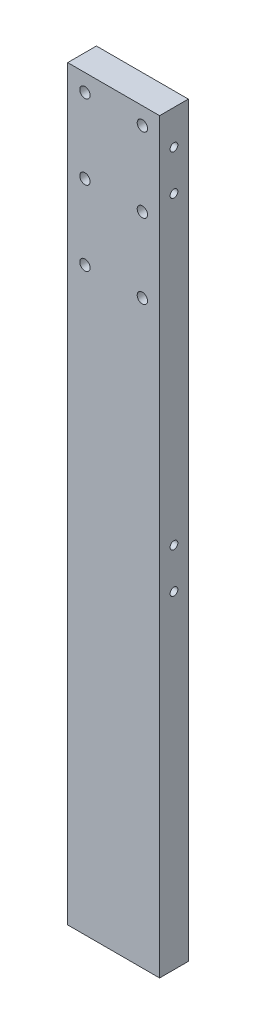
SolidWorks part; units mm, degrees
material "普通碳钢"
ref_plane "Front Plane" through (0, 0, 0) normal (0, 0, 1) x (1, 0, 0)
ref_plane "Top Plane" through (0, 0, 0) normal (0, 1, 0) x (1, 0, 0)
ref_plane "Right Plane" through (0, 0, 0) normal (1, 0, 0) x (0, 0, -1)
sketch "Sketch1" plane through (0, 0, 0) normal (0, 0, 1) x (1, 0, 0)
  line L0 (80, 0) -> (80, 80)
  line L1 (0, 0) -> (80, 0)
  line L2 (0, 0) -> (0, 650)
  line L3 (0, 650) -> (80, 650)
  line L5 (80, 80) -> (80, 650)
  dimension "D1" = 80
  dimension "D2" = 650
  dimension "D3" = 80
  dimension "D4" = 80
extrude "Boss-Extrude1" add sketch "Sketch1" along normal blind 25
hole_wizard "Ø9.0 (9) Diameter Hole1" positions "3DSketch1" profile "Sketch2" hole size "Ø9.0" standard "GB" end condition through all
sketch3d "3DSketch1"
  line L0 (15, 635, 25) -> (65, 635, 25) construction
  line L3 (65, 635, 25) -> (65, 505, 25) construction
  line L4 (65, 505, 25) -> (15, 505, 25) construction
  line L5 (15, 505, 25) -> (15, 635, 25) construction
  line L7 (40, 635, 25) -> (40, 650, 25) construction
  line L8 (80, 650, 25) -> (0, 650, 25) construction
  point P0 (15, 635, 25)
  point P2 (65, 635, 25)
  point P4 (15, 505, 25)
  point P6 (65, 505, 25)
  point P22 (15, 570, 25)
  point P24 (65, 570, 25)
  point P25 (15, 570, 25)
  point P27 (65, 570, 25)
  dimension "D1" = 130
  dimension "D2" = 50
  dimension "D3" = 15
  dimension "D4" = 65
sketch "Sketch2" plane through (15, 635, 25) normal (1, 0, 0) x (0, -1, 0)
  line L0 (0, 0) -> (0, 25)
  line L1 (0, 25) -> (4.5, 25)
  line L2 (4.5, 25) -> (4.5, 0)
  line L5 (4.5, 0) -> (0, 0)
  line L11 (0, -6.35) -> (0, 107.95) construction
  dimension "通孔孔直径" = 9
  dimension "通孔孔深度" = 25
hole_wizard "M8 Tapped Hole1" positions "Sketch3" profile "Sketch4" tap size "M8" standard "GB"
sketch "Sketch3" plane through (80, 500, 0) normal (1, 0, 0) x (0, -1, 0)
  line L0 (-102.5, 0) -> (-102.5, -25) construction
  line L8 (-150, -25) -> (-150, 0) construction
  line L9 (-150, -12.5) -> (73.142, -12.5) construction
  point P0 (-120, -12.5)
  point P2 (-85, -12.5)
  dimension "D1" = 35
  dimension "D2" = 47.5
sketch "Sketch4" plane through (80, 620, 12.5) normal (0, 1, 0) x (0, 0, -1)
  line L0 (0, 0) -> (0, 21.7929)
  line L1 (0, 21.7929) -> (3.4, 19.75)
  line L2 (3.4, 19.75) -> (3.4, 0)
  line L5 (3.4, 0) -> (0, 0)
  line L10 (0, 21.7929) -> (-3.4, 19.75) construction
  line L11 (0, -6.35) -> (0, 107.95) construction
  dimension "螺纹孔钻头直径" = 6.8
  dimension "螺纹孔钻头深度" = 19.75
  dimension "导头角度" = 118
cosmetic thread "Hole Cosmetic Thread1" parameters "D1"=16, "D2"=8
cosmetic thread "Hole Cosmetic Thread2" parameters "D1"=16, "D2"=8
pattern_linear "LPattern1" count 2 spacing 300 along (0, -1, 0) of "M8 Tapped Hole1"
cosmetic thread "Hole Cosmetic Thread3" parameters "D1"=16, "D2"=8
cosmetic thread "Hole Cosmetic Thread4" parameters "D1"=16, "D2"=8
